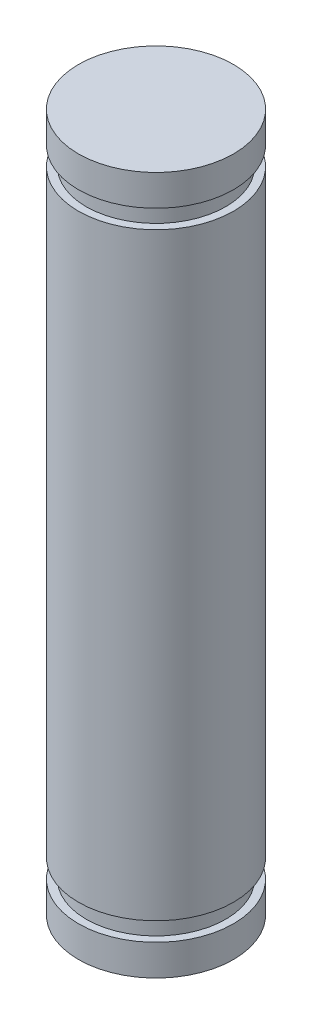
SolidWorks part; units mm, degrees
ref_plane "前视基准面" through (0, 0, 0) normal (0, 0, 1) x (1, 0, 0)
ref_plane "上视基准面" through (0, 0, 0) normal (0, 1, 0) x (1, 0, 0)
ref_plane "右视基准面" through (0, 0, 0) normal (1, 0, 0) x (0, 0, -1)
ref_plane "基准面4" through (0, 0, 0) normal (0, 0, -1) x (-1, 0, 0)
sketch "草图1" plane through (0, 0, 0) normal (0, 0, -1) x (-1, 0, 0)
  line L0 (-5, -22.5) -> (0, -22.5)
  line L1 (0, -22.5) -> (0, 22.5)
  line L2 (0, 22.5) -> (-5, 22.5)
  line L3 (-5, 22.5) -> (-5, 20.5)
  line L4 (-5, 20.5) -> (-4.5, 20.5)
  line L5 (-4.5, 20.5) -> (-4.5, 19.3)
  line L6 (-4.5, 19.3) -> (-5, 19.3)
  line L7 (-5, 19.3) -> (-5, -19.3)
  line L8 (-5, -19.3) -> (-4.5, -19.3)
  line L9 (-4.5, -19.3) -> (-4.5, -20.5)
  line L10 (-4.5, -20.5) -> (-5, -20.5)
  line L11 (-5, -20.5) -> (-5, -22.5)
  line L12 (0, -22.5) -> (0, 22.5) construction
revolve "旋转1" add sketch "草图1" angle 360 about L12
